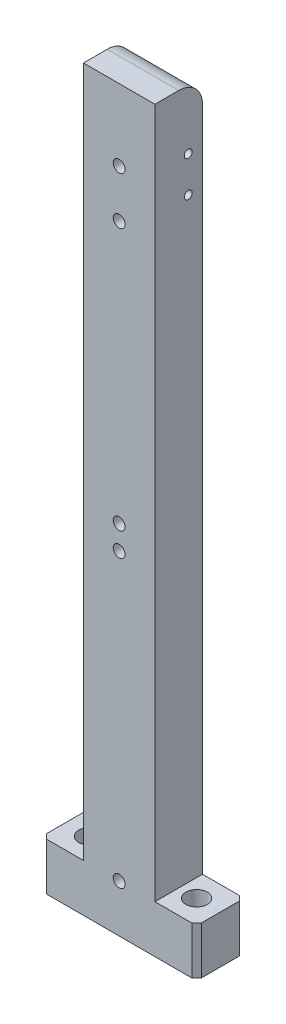
SolidWorks part; units mm, degrees
material "A6061"
ref_plane "前基準面" through (0, 0, 0) normal (0, 0, 1) x (1, 0, 0)
ref_plane "上基準面" through (0, 0, 0) normal (0, 1, 0) x (1, 0, 0)
ref_plane "右基準面" through (0, 0, 0) normal (1, 0, 0) x (0, 0, -1)
sketch "草图1" plane through (0, 0, 0) normal (0, 0, 1) x (1, 0, 0)
  line L0 (0, -1642.2848) -> (0, 80471.9574) construction
  line L1 (15, 310) -> (-15, 310)
  line L2 (-15, 310) -> (-15, 20)
  line L3 (-15, 20) -> (-32.5, 20)
  line L4 (-32.5, 20) -> (-32.5, 0)
  line L5 (-32.5, 0) -> (32.5, 0)
  line L6 (32.5, 20) -> (32.5, 0)
  line L7 (15, 20) -> (32.5, 20)
  line L8 (15, 310) -> (15, 20)
  point P10 (0, 0)
  point P13 (0, 310)
  dimension "D1" = 30
  dimension "D2" = 65
  dimension "D3" = 20
  dimension "D4" = 310
extrude "凸台-拉伸1" add sketch "草图1" along normal blind 20
hole_wizard "Ø9.0 (9) 直径孔1" positions "草图3" profile "草图2" hole size "Ø9.0" standard "GB" end condition through all
sketch "草图3" plane through (0, 20, 0) normal (0, 1, 0) x (1, 0, 0)
  line L0 (-32.5, -10) -> (32.5, -10) construction
  line L1 (-32.5, -20) -> (-32.5, 0) construction
  line L2 (32.5, -20) -> (32.5, 0) construction
  line L4 (0, -1000) -> (0, 49000) construction
  point P0 (22.5, -10)
  point P3 (-22.5, -10)
  dimension "D1" = 45
sketch "草图2" plane through (22.5, 20, 10) normal (1, 0, 0) x (0, 0, 1)
  line L0 (0, 0) -> (0, 20)
  line L1 (0, 20) -> (4.5, 20)
  line L2 (4.5, 20) -> (4.5, 0)
  line L5 (4.5, 0) -> (0, 0)
  line L11 (0, -6.35) -> (0, 107.95) construction
  dimension "通孔孔直径" = 9
  dimension "通孔孔深度" = 20
hole_wizard "M6 螺纹孔1" positions "草图5" profile "草图4" tap size "M6" standard "GB" end condition through all
sketch "草图5" plane through (0, 0, 20) normal (0, 0, 1) x (1, 0, 0)
  line L0 (-32.5, 0) -> (32.5, 0) construction
  line L1 (15, 310) -> (-15, 310) construction
  point P0 (0, 280)
  point P3 (0, 150)
  point P6 (0, 20)
  point P16 (0, 260)
  point P18 (0, 140)
  dimension "D1" = 20
  dimension "D2" = 130
  dimension "D3" = 130
  dimension "D4" = 50
  dimension "D5" = 120
sketch "草图4" plane through (0, 280, 20) normal (1, 0, 0) x (0, -1, 0)
  line L0 (0, 0) -> (0, 20)
  line L1 (0, 20) -> (2.5, 20)
  line L2 (2.5, 20) -> (2.5, 0)
  line L5 (2.5, 0) -> (0, 0)
  line L11 (0, -6.35) -> (0, 107.95) construction
  dimension "通孔螺纹孔钻头直径" = 5
  dimension "通孔螺纹孔钻头深度" = 20
cosmetic thread "孔螺蚊线1"
cosmetic thread "孔螺蚊线2"
cosmetic thread "孔螺蚊线6"
cosmetic thread "孔螺蚊线7"
cosmetic thread "孔螺蚊线8"
fillet "圆角1" radius 10 1 edges at (0, 310, 0)
chamfer "倒角1" distance 2 angle 45 4 edges at (32.5, 10, 20) (32.5, 10, 0) (-32.5, 10, 20) (-32.5, 10, 0)
hole_wizard "M4 螺纹孔1" positions "草图7" profile "草图6" tap size "M4" standard "GB" end condition through all
sketch "草图7" plane through (-15, 0, 0) normal (-1, 0, 0) x (0, 0, 1)
  line L0 (20, 310) -> (10, 310) construction
  line L1 (0, 300) -> (0, 20) construction
  point P0 (6, 285)
  point P2 (6, 270)
  dimension "D1" = 15
  dimension "D2" = 25
  dimension "D3" = 6
sketch "草图6" plane through (-15, 285, 6) normal (0, 1, 0) x (0, 0, 1)
  line L0 (0, 0) -> (0, 47.5)
  line L1 (0, 47.5) -> (1.65, 47.5)
  line L2 (1.65, 47.5) -> (1.65, 0)
  line L5 (1.65, 0) -> (0, 0)
  line L11 (0, -6.35) -> (0, 107.95) construction
  dimension "通孔螺纹孔钻头直径" = 3.3
  dimension "通孔螺纹孔钻头深度" = 47.5
cosmetic thread "孔螺蚊线4"
cosmetic thread "孔螺蚊线5"
